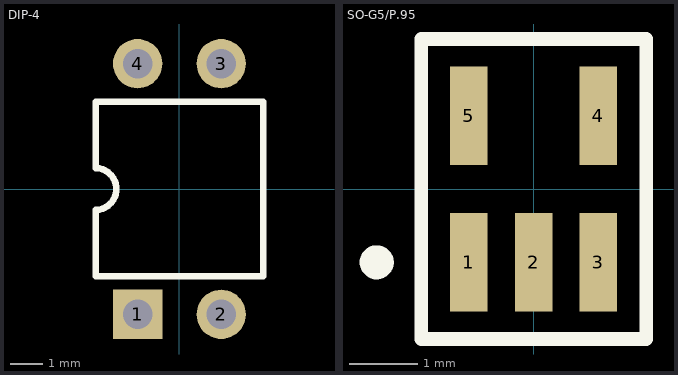
[diagram p0: the footprints below, top view; thin cyan lines are the x and y axes]
# Altium footprint library MISC95141-3.PCBLIB: 2 footprints
Each footprint in its own frame and in the unit in brackets; x right, y up, seen from the top. Pads: shape width x height; smd on the part's side, far side on the other; paste and mask are expansions set on the pad; w line width, h text height; cw(c..) or ccw(c..) is an arc to the next point about the centre after c.

## DIP-4 [mm]
pads (4):
  rect 1.5x1.5 hole 0.9: 1(-1.27,-3.81)
  round 1.5 hole 0.9: 2(1.27,-3.81) 3(1.27,3.81) 4(-1.27,3.81)
Top Overlay:
  lines w0.2: -2.55,-2.65 -2.55,-0.635 ccw(c-2.55,0) -2.55,0.635 -2.55,2.65 2.55,2.65 2.55,-2.65 -2.55,-2.65

## SO-G5/P.95 [mm]
pads (5):
  rect 0.55x1.45 smd: 1(-0.95,-1.075) 2(0,-1.075) 3(0.95,-1.075) 4(0.95,1.075) 5(-0.95,1.075)
Top Overlay:
  circle w0.25: c-2.3,-1.075 r0.125
  lines w0.2: -1.65,-2.2 -1.65,2.2 1.65,2.2 1.65,-2.2 -1.65,-2.2